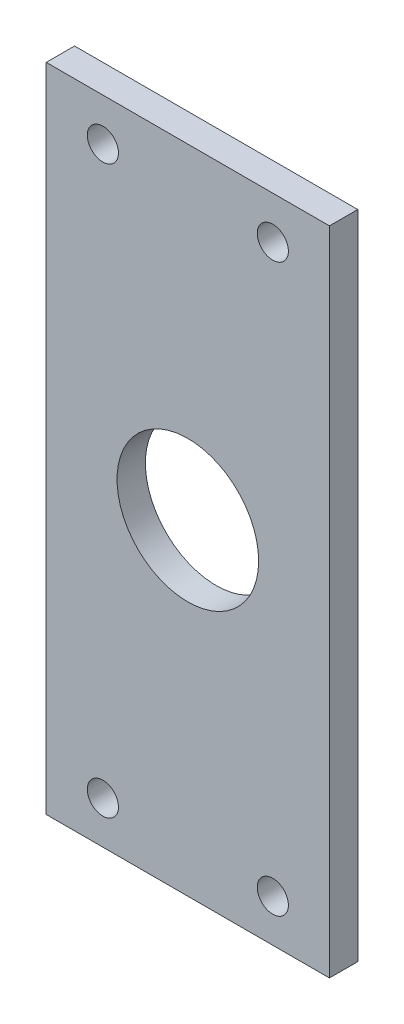
from build123d import *

# Parameters (mm, degrees)
SKETCH_1_W          = 100
SKETCH_1_H          = 230
SKETCH_1_R          = 25
SKETCH_1_R_2        = 5.5
BOSS_EXTRUDE1_DEPTH = 10


with BuildPart() as part:
    # Sketch 1 → Boss-Extrude1 (new body)
    with BuildSketch(Plane.XY):
        Rectangle(SKETCH_1_W, SKETCH_1_H)
        Circle(SKETCH_1_R, mode=Mode.SUBTRACT)
        with Locations((-30, 100)):
            Circle(SKETCH_1_R_2, mode=Mode.SUBTRACT)
        with Locations((30, 100)):
            Circle(SKETCH_1_R_2, mode=Mode.SUBTRACT)
        with Locations((30, -100)):
            Circle(SKETCH_1_R_2, mode=Mode.SUBTRACT)
        with Locations((-30, -100)):
            Circle(SKETCH_1_R_2, mode=Mode.SUBTRACT)
    extrude(amount=BOSS_EXTRUDE1_DEPTH)


solid = part.part
